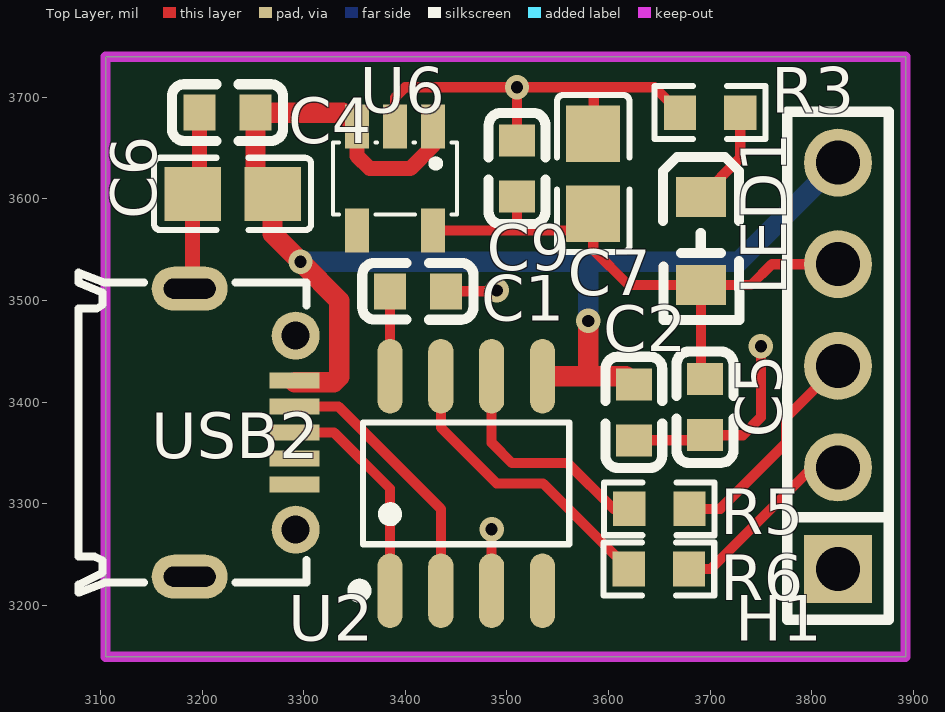
[diagram p0: Top Layer view]
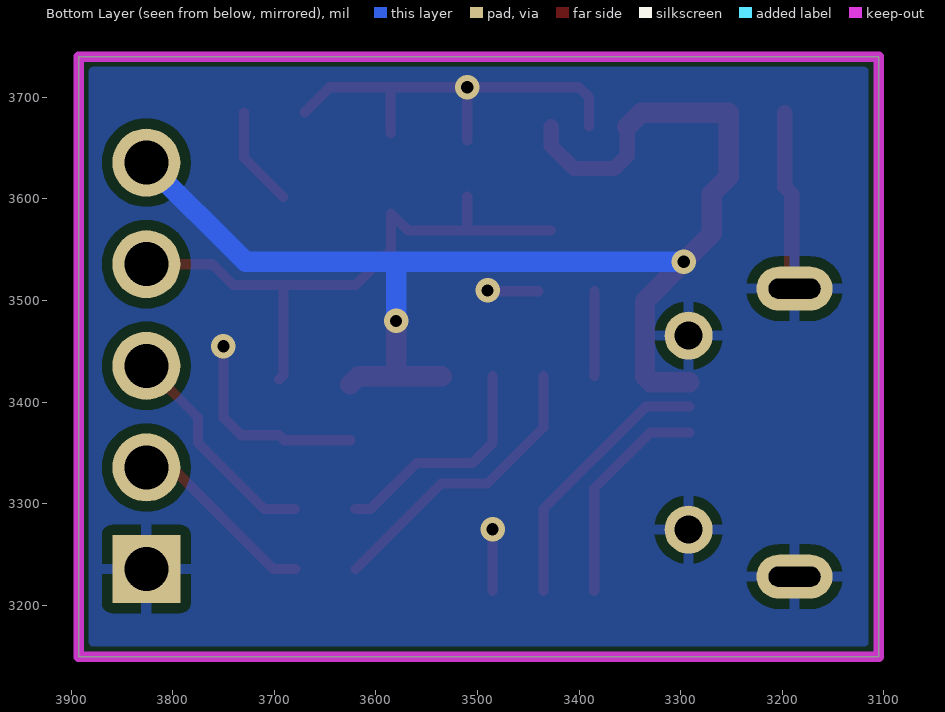
[diagram p1: Bottom Layer view, seen from below]
# Altium PCB MISC89035.pcbdoc
Units mil, origin at the board's own origin, x right, y up, seen from the top; angles counter-clockwise.
Board outline 787.4 x 590.55 mil, 2 copper layers (Top Layer, Bottom Layer), stack 62.206 mil thick; 15 components, 11 nets, 49 pads, 6 vias.

## Layer stack, top to bottom
Top Solder Mask Layer: solder mask 0.394, Dk 3.3
Top Layer: signal copper 1.379
Dielectric1: surface 59.449, FR4, Dk 4.5
Bottom Layer: signal copper 1.378
Bottom Solder Mask Layer: solder mask 0.394, Dk 3.3

## Board outline
3105,3740 3105,3149.45 3892.4,3149.45 3892.4,3740

## Design rules (kind name [scope] priority, off if disabled: settings)
BoardOutlineClearance copperThickness2oz_1 [All] p2 off: genericclearance=7.99 ignorepadtopadclearanceinfootprint=FALSE except(0: Arc-SplitContinuation Track-SplitContinuation SMDPad-SplitContinuation THPad-SplitContinuation Via-SplitContinuation Fill-SplitContinuation Region-SplitContinuation Poly-SplitContinuation Text-SplitContinuation Hole-SplitContinuation; 5.98: Arc-CutoutEdge SMDPad-CutoutEdge THPad-CutoutEdge Via-CutoutEdge Fill-CutoutEdge Region-CutoutEdge Text-CutoutEdge; 6.93: Hole-OutlineEdge Hole-CutoutEdge; 10: Poly-OutlineEdge Poly-CutoutEdge; 11.81: Arc-OutlineEdge Track-OutlineEdge SMDPad-OutlineEdge THPad-OutlineEdge Via-OutlineEdge Fill-OutlineEdge Region-OutlineEdge Text-OutlineEdge Track-CutoutEdge)
BoardOutlineClearance copperThickness1oz_1 [All] p4: genericclearance=4.02 ignorepadtopadclearanceinfootprint=FALSE except(0: Arc-SplitContinuation Track-SplitContinuation SMDPad-SplitContinuation THPad-SplitContinuation Via-SplitContinuation Fill-SplitContinuation Region-SplitContinuation Poly-SplitContinuation Text-SplitContinuation Hole-SplitContinuation; 6: SMDPad-CutoutEdge THPad-CutoutEdge Via-CutoutEdge Fill-CutoutEdge Region-CutoutEdge Text-CutoutEdge; 6.93: Hole-OutlineEdge Hole-CutoutEdge; 10: Poly-OutlineEdge Poly-CutoutEdge; 11.8: Arc-OutlineEdge Track-OutlineEdge SMDPad-OutlineEdge THPad-OutlineEdge Via-OutlineEdge Fill-OutlineEdge Region-OutlineEdge Text-OutlineEdge; 11.81: Arc-CutoutEdge Track-CutoutEdge)
Clearance copperThickness2oz [All] p1 off: gap=7.99 ignorepadtopadclearanceinfootprint=FALSE except(5.98: SMDPad-Track SMDPad-SMDPad THPad-Track SMDPad-THPad THPad-THPad Track-Via SMDPad-Via THPad-Via Via-Via Fill-Track Region-Track Fill-SMDPad Region-SMDPad Fill-THPad Region-THPad Fill-Via Region-Via Fill-Fill Fill-Region Region-Region Arc-Track Arc-SMDPad Arc-THPad Arc-Via Fill-Arc Region-Arc Arc-Arc Text-Track SMDPad-Text Text-THPad Text-Via Fill-Text Region-Text Arc-Text Text-Text; 6.93: Hole-Track Hole-SMDPad Hole-THPad Hole-Via Fill-Hole Region-Hole Hole-Arc Hole-Text; 10: Poly-Track Poly-SMDPad Poly-THPad Poly-Via Poly-Fill Poly-Region Poly-Poly Poly-Arc Poly-Text Poly-Hole)
Clearance copperThickness1oz [All] p3: gap=4.02 ignorepadtopadclearanceinfootprint=FALSE except(5.98: SMDPad-Track SMDPad-SMDPad THPad-Track SMDPad-THPad THPad-THPad Track-Via SMDPad-Via THPad-Via Via-Via Fill-Track Region-Track Fill-SMDPad Region-SMDPad Fill-THPad Region-THPad Fill-Via Region-Via Fill-Fill Fill-Region Region-Region; 6: Arc-Track Arc-SMDPad Arc-THPad Arc-Via Fill-Arc Region-Arc Arc-Arc Text-Track SMDPad-Text Text-THPad Text-Via Fill-Text Region-Text Arc-Text Text-Text; 6.93: Hole-Track Hole-SMDPad Hole-THPad Hole-Via Fill-Hole Region-Hole Hole-Arc Hole-Text; 10: Poly-Track Poly-SMDPad Poly-THPad Poly-Via Poly-Fill Poly-Region Poly-Poly Poly-Arc Poly-Text Poly-Hole)
Creepage creepage [All] p1: checkdistance=0 ignoreinternallayers=TRUE applytopolygonpour=TRUE
DiffPairsRouting differentialPair [All] p1: maxlimit=6 minlimit=6 mostfreqgap=6 toplayer_minwidth=5 toplayer_prefwidth=10 toplayer_maxwidth=100 toplayer_mingap=6 toplayer_prefgap=6 toplayer_maxgap=6 bottomlayer_minwidth=5 bottomlayer_prefwidth=10 bottomlayer_maxwidth=100 bottomlayer_mingap=6 bottomlayer_prefgap=6 bottomlayer_maxgap=6 maxuncoupledlength=10
HoleToHoleClearance otherClearance [All] p1: gap=11.81 allowstackedmicrovias=TRUE
Length netLength [All] p1: minlimit=0 maxlimit=0
MatchedLengths netLengthTolerance [All] p1: tolerance=1000
PasteMaskExpansion pasteMaskExpansion [All] p1: expansion=0
PlaneConnect innerPlane [All] p1: planeconnectstyle=Relief reliefexpansion=20 reliefentries=4 reliefconductorwidth=10 reliefairgap=10
PolygonConnect copperRegion [(InNet('GND'))] p1: connectstyle=Relief reliefconductorwidth=10 reliefentries=4 polygonreliefangle="90 Angle" airgapwidth=10 via.connectstyle=Relief via.reliefconductorwidth=10 via.reliefentries=4 via.polygonreliefangle="90 Angle" via.airgapwidth=10
RoutingVias viaSize [All] p1: holewidth=12.01 width=24.02 viastyle="Through Hole" minholewidth=11.81 minwidth=19.68 maxholewidth=248.03 maxwidth=393.7
SolderMaskExpansion solderMaskExpansion [IsVia] p1: expansion=-1000 istentingtop=TRUE
SolderMaskExpansion solderMaskExpansion [All] p2: expansion=2 istentingtop=FALSE
Width copperThickness2oz_2 [All] p1 off: maxlimit=100 minlimit=8 preferedwidth=10
Width copperThickness1oz_2 [All] p2: maxlimit=100 minlimit=5 preferedwidth=10

## Components (designator, comment, footprint, x,y, rotation, side; value= is the part's Value field where it differs from the comment)
C1 "100nF" C0603 3412.36,3509.13 r180 top
C2 "100nF" C0603 3625,3390 r90 top
C4 "100nF" C0603 3225,3685 r0 top
C5 "100nF" C0603 3695,3395 r90 top
C6 "22uF" C0805 3230,3605 r0 top
C7 "22uF" C0805 3585,3625 r270 top
C9 "100nF" C0603 3510,3630 r270 top
H1 "PZ254V-11-05P" HDR-TH_5P-P2.54-V-M 3825.89,3435.78 r90 top
LED1 "NCD0805R1" LED0805-RD 3691,3558.67 r270 top
R3 "1kΩ" R0603 3700,3685 r0 top
R5 "22Ω" R0603 3650,3295 r0 top
R6 "22Ω" R0603 3649.54,3235.78 r0 top
U2 "CH340N" SOP-8_L4.9-W3.9-P1.27-LS6.0-BL 3460,3320 r0 top
U6 "XC6219B332MR" SOT-23-5_L3.0-W1.7-P0.95-LS2.8-BR 3390,3620 r90 top
USB2 "920-E52A2021S10100" MICRO-USB-SMD_5P-P0.65-H-F_C10418 3240,3370 r270 top

## Footprints (in the part's own frame and the unit in brackets; to place one, negate y for a bottom-side part, rotate by r counter-clockwise, add the part's x,y. Pads: shape width x height; smd on the part's side, far side on the other; paste and mask are expansions set on the pad)
C0603 [mm]
  rect 0.8x0.9 smd: 1(-0.7,0) 2(0.7,0)
  silkscreen extent -1.39,-0.71 1.39,0.71
C0805 [mm]
  rect 1.41x1.35 smd paste-100 mask+0.051: 1(-1,0) 2(1,0)
  silkscreen extent -1.96,-0.9 1.96,0.9
HDR-TH_5P-P2.54-V-M [mm]
  rect 1.7x1.7 hole 1.1: 1(-5.08,0)
  round 1.7 hole 1.1: 2(-2.54,0) 3(0,0) 4(2.54,0) 5(5.08,0)
  silkscreen extent -6.35,-1.27 6.35,1.27
LED0805-RD [mm]
  rect 1x1.25 smd: 1(-1.1,0) 2(1.1,0)
  silkscreen extent -2.1,-0.95 1.98,0.96
MICRO-USB-SMD_5P-P0.65-H-F_C10418 [mm]
  rect 0.4x1.25 smd paste-100 mask+0.05: 1(-1.3,1.3) 2(-0.65,1.3) 3(0,1.3) 4(0.65,1.3) 5(1.3,1.3)
  round 1.2 hole 0.7 paste+0 mask+0.05: SH0(-2.425,1.325) SH3(2.425,1.325)
  oval 1.1x1.9 hole 0.5 slot 1.3 at 90 deg: SH1(-3.6,-1.325) SH2(3.6,-1.325)
  silkscreen extent -4,-4.1 4,1.6
R0603 [mil]
  rect 31.75x34.02 smd paste-3937.01 mask+2: 1(-29.66,0) 2(29.66,0)
  silkscreen extent -55,-26 55,26
SOP-8_L4.9-W3.9-P1.27-LS6.0-BL [mm]
  oval 0.63x1.865 smd: 1(-1.905,-2.682) 2(-0.635,-2.682) 3(0.635,-2.682) 4(1.905,-2.682) 5(1.905,2.682) 6(0.635,2.682) 7(-0.635,2.682) 8(-1.905,2.682)
  silkscreen extent -2.82,-2.83 2.58,1.52
SOT-23-5_L3.0-W1.7-P0.95-LS2.8-BR [mm]
  rect 1.1x0.6 smd: 1(1.3,-0.95) 2(1.3,0) 3(1.3,0.95) 4(-1.3,0.95) 5(-1.3,-0.95)
  silkscreen extent -0.9,-1.55 0.9,1.55

## Via types
v1: diameter 24.02, hole 12, Top Layer to Bottom Layer, 6 vias

## Nets (pads, with @x,y where several pads share a name; then routed paths per layer and width w, separated by ;. In a path a pad name is that pad's centre, name@x,y a point inside that pad or via, vN(x,y) a via of type N, cw(c..) or ccw(c..) an arc to the next point about the centre after c; other vN are vias at no path point)
3V3: C5.2 C7.2 C9.2 H1.4 LED1.2 U6.5 | length 592.2
  Top Layer w10: U6.5 3509.44,3568.82 ; C9.2 3510,3569.37 3509.44,3568.82 ; C5.2 3691,3426.56 LED1.2 ; H1.4 3760.78,3535.78 3740.36,3515.36 LED1.2 ; 3509.44,3568.82 3568.18,3568.82 C7.2 3585,3550 3619.64,3515.36 LED1.2
5V: C2.2 C4.2 C6.2 H1.5 U2.5 U6.1 U6.3 USB2.1 | length 1358.6
  Top Layer w15: U6.3 3352.6,3642.4 3365,3630 3405,3630 3427.4,3652.4 U6.1
  Top Layer w20: USB2.1@3291.17,3419.45 3329.45,3419.45 3335,3425 3335,3500 v1(3296.88,3538.12) 3269.37,3565.63 C6.2 3252.56,3621.81 C4.2 3338.78,3685 U6.3 ; U2.5 3581.02,3425.61 ; v1(3580,3480) 3580,3426.63 3581.02,3425.61 ; C2.2 3616.95,3425.61 3581.02,3425.61
  Bottom Layer w20: v1(3296.88,3538.12) 3580,3538.12 ; v1(3580,3480) 3580,3538.12 ; H1.5 3728.23,3538.12 3580,3538.12
$1N10: LED1.1 R3.2 | length 99
  Top Layer w10: LED1.1 3729.66,3640.64 R3.2
$1N19: C1.2 U2.8 | length 83.6
  Top Layer w10: C1.2 3384.8,3425.81 U2.8
$1N20: R5.1 U2.6 | length 227.9
  Top Layer w10: U2.6 3485,3360 3505,3340 3560,3340 3605,3295 R5.1
$1N21: R6.1 U2.7 | length 293.2
  Top Layer w10: U2.7 3435,3375 3490,3320 3535.67,3320 R6.1
$1N22: H1.3 R5.2 | length 219.1
  Top Layer w10: R5.2 3710,3295 3775,3360 3775,3384.89 H1.3
$1N23: H1.2 R6.2 | length 188.1
  Top Layer w10: R6.2 3700.78,3235.78 3800.78,3335.78 H1.2
$1N29: U2.2 USB2.2 | length 266.1
  Top Layer w10: USB2.2 3334.41,3395.59 3435,3295 U2.2
$1N30: U2.1 USB2.3 | length 217.2
  Top Layer w10: USB2.3 3330,3370 3385,3315 U2.1
GND: C1.1 C2.1 C4.1 C5.1 C6.1 C7.1 C9.1 H1.1 R3.1 U2.3 U6.2 USB2.SH0 USB2.SH1 USB2.SH2 USB2.SH3 | length 914.6
  Top Layer w10: U6.2 3390,3700 3400,3710 v1(3510,3710) ; C1.1 3489.13,3509.13 v1(3490,3510) ; U2.3 v1(3485,3275) ; C9.1 v1(3510,3710) ; C7.1 3585.5,3664.87 3585.5,3710 ; C2.1 3690,3362.44 C5.1 3732.44,3367.44 3750,3385 v1(3750,3455) ; R3.1 3645.34,3710 3585.5,3710 ; v1(3510,3710) 3585.5,3710
  Top Layer w15: USB2.SH1 3190.63,3514.53 C6.1 3197.44,3611.81 C4.1
pads on no net: U2.4 U6.4 USB2.4 USB2.5

## Polygon pours and split planes (outlines as drawn)
GND on Bottom Layer (solid, remove dead copper, pour order 0): 3000,3785 3000,3000 4005,3000 4005,3785

## Keep-outs
Board Outline Layer:
  the board outline again, w10